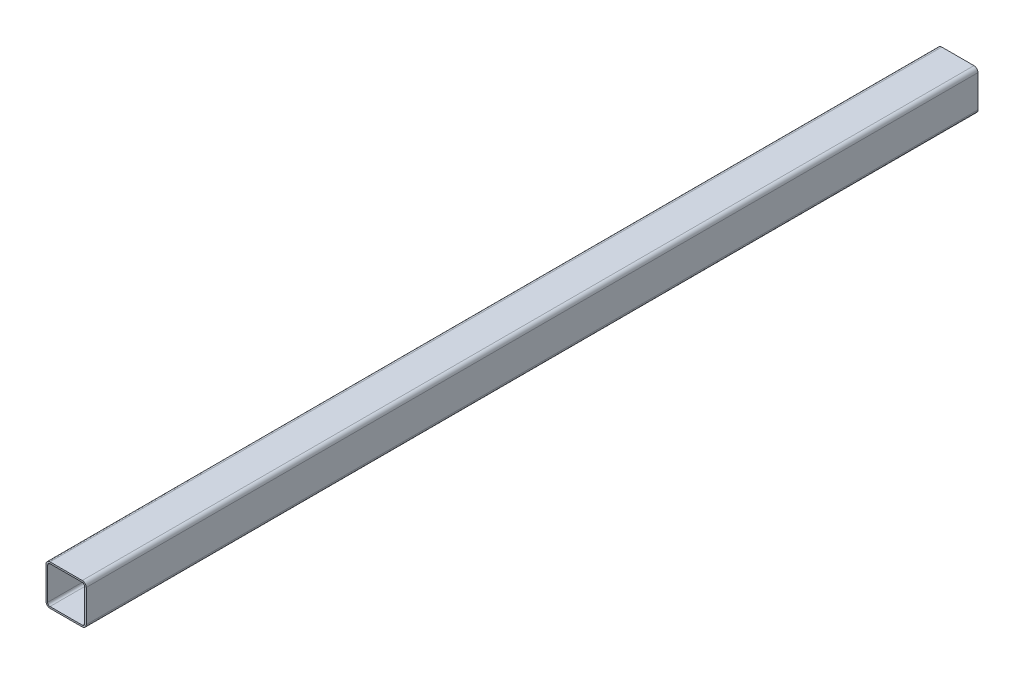
from build123d import *

# Parameters (mm, degrees)
BOSS_EXTRUDE1_DEPTH = 4430


with BuildPart() as part:
    # Sketch1 → Boss-Extrude1 (new body)
    with BuildSketch(Plane.XY):
        with BuildLine():
            Line((-80, 100), (80, 100))
            ThreePointArc((80, 100), (94.142135624, 94.142135624), (100, 80))
            Line((100, 80), (100, -80))
            ThreePointArc((100, -80), (94.142135624, -94.142135624), (80, -100))
            Line((80, -100), (-80, -100))
            ThreePointArc((-80, -100), (-94.142135624, -94.142135624), (-100, -80))
            Line((-100, -80), (-100, 80))
            ThreePointArc((-100, 80), (-94.142135624, 94.142135624), (-80, 100))
        make_face()
        with BuildLine():
            Line((-92, 80), (-92, -80))
            ThreePointArc((-92, -80), (-88.485281374, -88.485281374), (-80, -92))
            Line((-80, -92), (80, -92))
            ThreePointArc((80, -92), (88.485281374, -88.485281374), (92, -80))
            Line((92, -80), (92, 80))
            ThreePointArc((92, 80), (88.485281374, 88.485281374), (80, 92))
            Line((80, 92), (-80, 92))
            ThreePointArc((-80, 92), (-88.485281374, 88.485281374), (-92, 80))
        make_face(mode=Mode.SUBTRACT)
    extrude(amount=BOSS_EXTRUDE1_DEPTH)


solid = part.part
